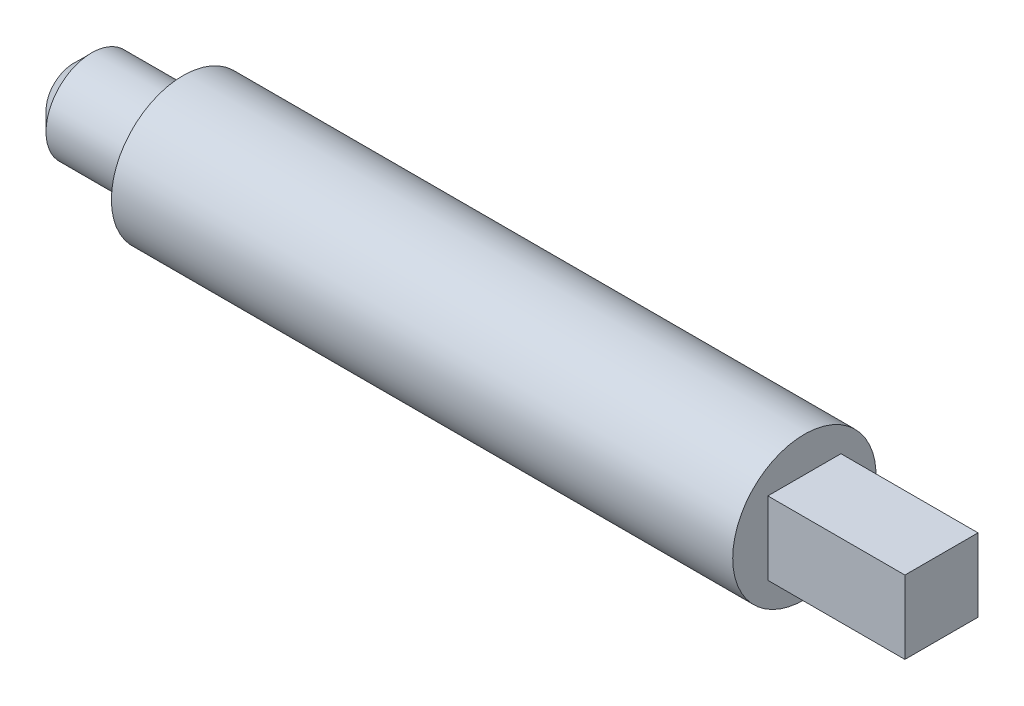
SolidWorks part; units mm, degrees
ref_plane "Front Plane" through (0, 0, 0) normal (0, 0, 1) x (1, 0, 0)
ref_plane "Top Plane" through (0, 0, 0) normal (0, 1, 0) x (1, 0, 0)
ref_plane "Right Plane" through (0, 0, 0) normal (1, 0, 0) x (0, 0, -1)
sketch "Sketch1" plane through (0, 0, 0) normal (0, 0, 1) x (1, 0, 0)
  line L0 (0, 0) -> (80, 0) construction
  line L1 (0, 0) -> (0, 5)
  line L2 (0, 5) -> (12, 5)
  line L3 (12, 5) -> (12, 7.845)
  line L4 (12, 7.845) -> (80, 7.845)
  line L5 (80, 7.845) -> (80, 0)
  line L6 (0, 0) -> (80, 0)
  dimension "D1" = 80
  dimension "D2" = 7.845
  dimension "D3" = 5
  dimension "D4" = 12
revolve "Revolve1" add sketch "Sketch1" angle 360 about L0
sketch "Sketch2" plane through (80, 0, 0) normal (1, 0, 0) x (0, 0, -1)
  line L1 (-4, -4) -> (4, -4)
  line L2 (-4, -4) -> (-4, 4)
  line L3 (-4, 4) -> (4, 4)
  line L4 (4, -4) -> (4, 4)
  line L5 (-4, -4) -> (4, 4) construction
  line L6 (-4, 4) -> (4, -4) construction
  point P0 (0, 0)
  dimension "D1" = 8
  dimension "D2" = 8
extrude "Boss-Extrude1" add sketch "Sketch2" along normal blind 15
chamfer "Chamfer1" distance 2 angle 45 1 edges at (0, 0, 5)
